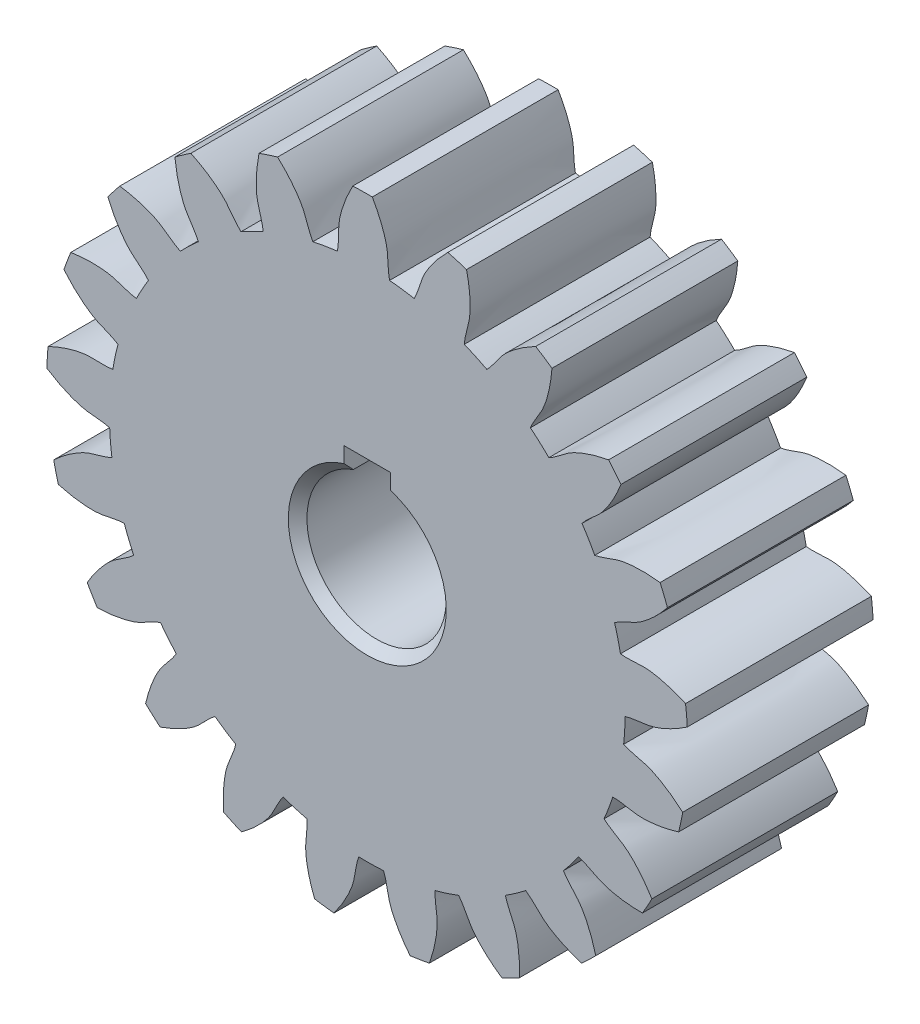
SolidWorks part; units mm, degrees
material "45"
ref_plane "Front Plane" through (0, 0, 0) normal (0, 0, 1) x (1, 0, 0)
ref_plane "Top Plane" through (0, 0, 0) normal (0, 1, 0) x (1, 0, 0)
ref_plane "Right Plane" through (0, 0, 0) normal (1, 0, 0) x (0, 0, -1)
sketch "Sketch1" plane through (0, 0, 0) normal (0, 0, 1) x (1, 0, 0)
  circle A0 centre (0, 0) radius 27.75
  circle A1 centre (0, 0) radius 7.5
  dimension "D1" = 55.5
  dimension "D2" = 15
extrude "Boss-Extrude1" add sketch "Sketch1" along normal blind 20
sketch "Sketch2" plane through (0, 0, 0) normal (0, 0, 1) x (1, 0, 0)
  arc A0 (34.2512, 4.1358) -> (34.4395, 2.0426) centre (0, 0) cw
  arc A1 (27.245, 5.27) -> (27.7481, -0.3236) centre (0, 0) cw
  spline S0 degree 3 poles (34.4395, 2.0426) (33.8282, 1.6273) (32.8868, 1.0623) (31.5721, 0.4842) (30.0037, -0.0651) (28.6639, -0.0376) (27.7481, -0.3236) knots 0 0 0 0 0.308946 0.45663 0.599771 1 1 1 1
  spline S1 degree 3 poles (34.2512, 4.1358) (33.5757, 4.4354) (32.5485, 4.8233) (31.1518, 5.1576) (29.5105, 5.4181) (28.1972, 5.152) (27.245, 5.27) knots 0 0 0 0 0.308946 0.45663 0.599771 1 1 1 1
extrude "Boss-Extrude2" add sketch "Sketch2" along normal blind 20
pattern_circular "CirPattern1" count 21 over 360 about axis through (0, 0, 20) along (0, 0, -1) of "Boss-Extrude2"
chamfer "Chamfer1" distance 1 angle 45 2 edges at (7.5, 0, 0) (7.5, 0, 20)
sketch "Sketch3" plane through (0, 0, 20) normal (0, 0, 1) x (1, 0, 0)
  line L1 (2.5, 5.2) -> (-2.5, 5.2)
  line L2 (2.5, 5.2) -> (2.5, 9.8)
  line L3 (2.5, 9.8) -> (-2.5, 9.8)
  line L4 (-2.5, 5.2) -> (-2.5, 9.8)
  line L5 (2.5, 5.2) -> (-2.5, 9.8) construction
  line L6 (2.5, 9.8) -> (-2.5, 5.2) construction
  circle A0 centre (0, 0) radius 7.5 construction
  point P0 (0, 7.5)
  dimension "D1" = 17.3
  dimension "D2" = 5
extrude "Cut-Extrude1" cut sketch "Sketch3" against normal up to next
